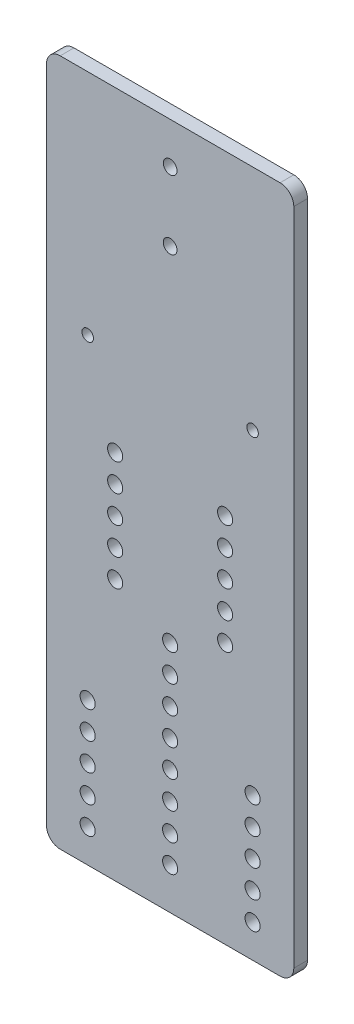
from build123d import *

# Parameters (mm, degrees)
SKETCH_1_W          = 90
SKETCH_1_H          = 250
EXTRUDE_1_DEPTH     = 5
SKETCH_2_R          = 2.5
SKETCH_2_R_2        = 2.1
CUT_EXTRUDE_1_DEPTH = 5
SKETCH_3_R          = 2.75
CUT_EXTRUDE_2_DEPTH = 5
SKETCH_4_R          = 2.75
CUT_EXTRUDE_3_DEPTH = 5
FILLET_1_R          = 5


with BuildPart() as part:
    # 草图1 → 凸台-拉伸1 (new body)
    with BuildSketch(Plane.XY):
        Rectangle(SKETCH_1_W, SKETCH_1_H)
    extrude(amount=EXTRUDE_1_DEPTH)

    # 草图2 → 切除-拉伸1 (cut)
    with BuildSketch(Plane.XY.offset(5)):
        with Locations((0, 110)):
            Circle(SKETCH_2_R)
        with Locations((0, 85)):
            Circle(SKETCH_2_R)
        with Locations((-30, 42)):
            Circle(SKETCH_2_R_2)
        with Locations((30, 42)):
            Circle(SKETCH_2_R_2)
    extrude(amount=-CUT_EXTRUDE_1_DEPTH, mode=Mode.SUBTRACT)

    # 草图3 → 切除-拉伸2 (cut)
    with BuildSketch(Plane.XY.offset(5)):
        with Locations((-20, -30)):
            Circle(SKETCH_3_R)
        with Locations((20, -30)):
            Circle(SKETCH_3_R)
        with Locations((0, -80)):
            Circle(SKETCH_3_R)
        with Locations((0, -70)):
            Circle(SKETCH_3_R)
        with Locations((0, -60)):
            Circle(SKETCH_3_R)
        with Locations((0, -50)):
            Circle(SKETCH_3_R)
        with Locations((0, -40)):
            Circle(SKETCH_3_R)
        with Locations((0, -90)):
            Circle(SKETCH_3_R)
        with Locations((0, -100)):
            Circle(SKETCH_3_R)
        with Locations((0, -110)):
            Circle(SKETCH_3_R)
        with Locations((-20, -20)):
            Circle(SKETCH_3_R)
        with Locations((20, -20)):
            Circle(SKETCH_3_R)
        with Locations((-20, -10)):
            Circle(SKETCH_3_R)
        with Locations((20, -10)):
            Circle(SKETCH_3_R)
        with Locations((-20, 0)):
            Circle(SKETCH_3_R)
        with Locations((20, 0)):
            Circle(SKETCH_3_R)
        with Locations((-20, 10)):
            Circle(SKETCH_3_R)
        with Locations((20, 10)):
            Circle(SKETCH_3_R)
    extrude(amount=-CUT_EXTRUDE_2_DEPTH, mode=Mode.SUBTRACT)

    # 草图4 → 切除-拉伸3 (cut)
    with BuildSketch(Plane.XY.offset(5)):
        with Locations((-30, -113)):
            Circle(SKETCH_4_R)
        with Locations((30, -113)):
            Circle(SKETCH_4_R)
        with Locations((-30, -103)):
            Circle(SKETCH_4_R)
        with Locations((30, -103)):
            Circle(SKETCH_4_R)
        with Locations((-30, -93)):
            Circle(SKETCH_4_R)
        with Locations((30, -93)):
            Circle(SKETCH_4_R)
        with Locations((-30, -83)):
            Circle(SKETCH_4_R)
        with Locations((30, -83)):
            Circle(SKETCH_4_R)
        with Locations((-30, -73)):
            Circle(SKETCH_4_R)
        with Locations((30, -73)):
            Circle(SKETCH_4_R)
    extrude(amount=-CUT_EXTRUDE_3_DEPTH, mode=Mode.SUBTRACT)

    # 圆角1
    fillet_1_edges = [part.edges().sort_by_distance(p)[0] for p in [
        (45, -125, 2.5),
        (-45, -125, 2.5),
        (-45, 125, 2.5),
        (45, 125, 2.5),
    ]]
    fillet(fillet_1_edges, radius=FILLET_1_R)


solid = part.part
